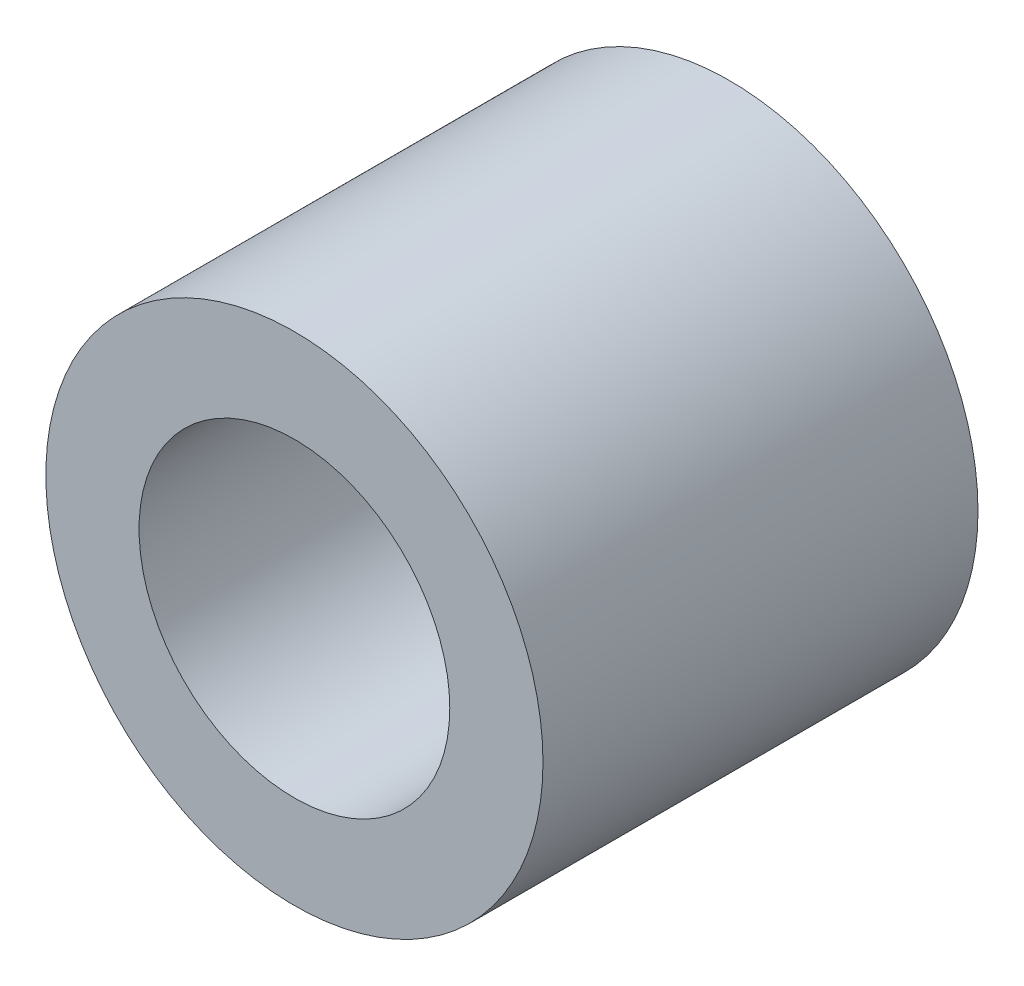
from build123d import *

# Parameters (mm, degrees)
SKETCH_1_R      = 4
SKETCH_1_R_2    = 2.5
EXTRUDE_1_DEPTH = 7


with BuildPart() as part:
    # 草图1 → 凸台-拉伸1 (new body)
    with BuildSketch(Plane.XY):
        Circle(SKETCH_1_R)
        Circle(SKETCH_1_R_2, mode=Mode.SUBTRACT)
    extrude(amount=EXTRUDE_1_DEPTH)


solid = part.part
